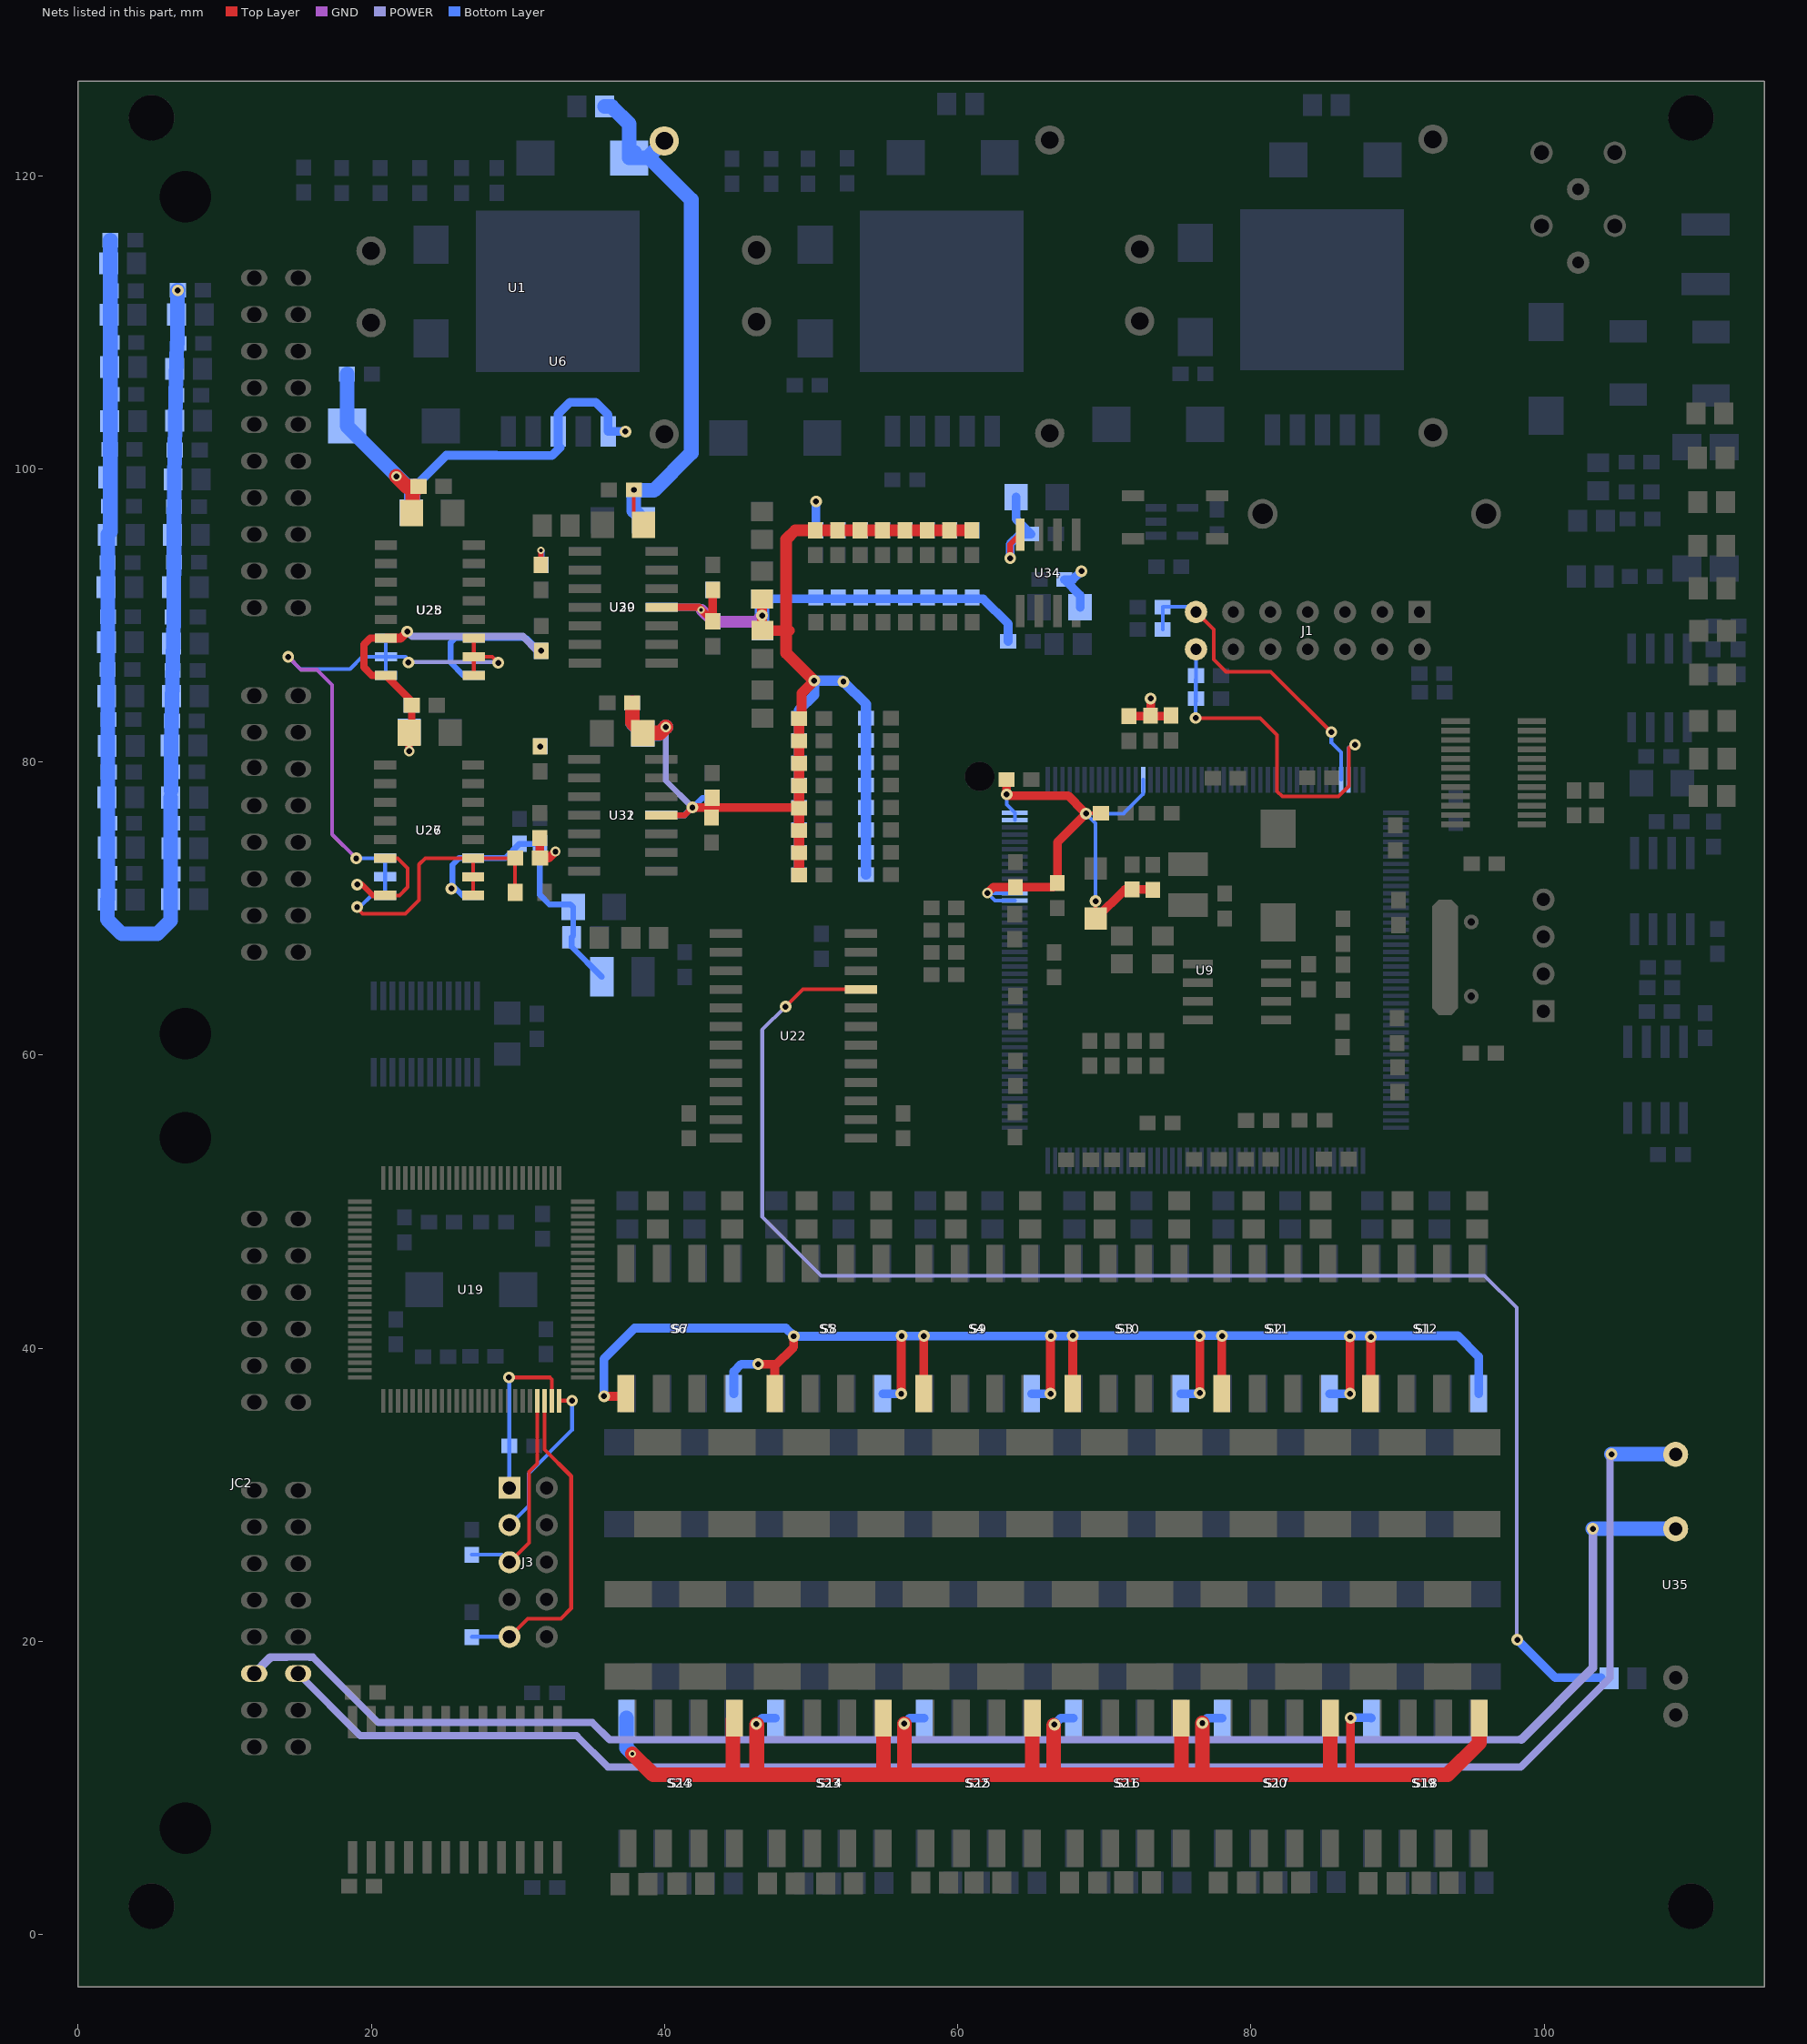
[diagram p0: the nets of this part, all layers, seen from the top]
# Altium PCB MISC86180.PCBDOC (part 6 of 9)
Units mm, origin at the board's own origin, x right, y up, seen from the top; angles counter-clockwise.
Board outline 115 x 130 mm, 4 copper layers (Top Layer, GND, POWER, Bottom Layer); 475 components, 355 nets, 1755 pads, 459 vias.

## Via types
v1: diameter 0.8, hole 0.4, Top Layer to Bottom Layer, 339 vias
v2: diameter 0.7, hole 0.4, Top Layer to Bottom Layer, 83 vias
v3: diameter 0.5, hole 0.254, Top Layer to Bottom Layer, 37 vias

## Nets (pads, with @x,y where several pads share a name; then routed paths per layer and width w, separated by ;. In a path a pad name is that pad's centre, name@x,y a point inside that pad or via, vN(x,y) a via of type N, cw(c..) or ccw(c..) an arc to the next point about the centre after c; other vN are vias at no path point) (continued)
CT26: R104.2 U22.9 | length 104
  Top Layer w0.254: v1(48.25,63.31) 49.429,64.489 U22.9@53.392,64.489
  POWER w0.254: v1(48.25,63.31) 46.66,61.72 46.66,48.99 50.69,44.96 95.92,44.96 98.11,42.77 v1@98.11,20.11
  Bottom Layer w0.6: v1@98.19,20.09 100.74,17.54 R104.2@103.879,17.54
  other v1: 98.16,20.12
CTCK: J3.1 R83.2 U19.24 | length 12
  Top Layer w0.254: v1(29.39,38.01) 32.19,38.01 32.316,37.884 U19.24@32.316,36.414
  Bottom Layer w0.254: v1(29.39,38.01) 29.41,37.99 R83.2@29.41,33.332 J3.1@29.41,30.5
CTDI: J3.9 R85.2 U19.23 | length 22.5
  Top Layer w0.254: J3.9@29.425,20.325 30.659,21.56 32.93,21.56 33.63,22.26 33.63,31.28 31.816,33.094 U19.23@31.816,36.414
  Bottom Layer w0.254: R85.2@26.848,20.3 26.874,20.325 J3.9@29.425,20.325
CTDO: J3.3 U19.25 | length 11.1
  Top Layer w0.254: U19.25@32.816,36.414 32.832,36.43 v1(33.69,36.43)
  Bottom Layer w0.254: J3.3@29.425,27.945 30.719,29.24 30.719,31.46 33.69,34.431 v1(33.69,36.43)
CTMS: J3.5 R84.2 U19.22 | length 14.6
  Top Layer w0.254: J3.5@29.425,25.405 30.76,26.741 30.76,31.58 31.316,32.136 U19.22@31.316,36.414
  Bottom Layer w0.254: R84.2@26.848,25.92 28.91,25.92 J3.5@29.425,25.405
CTOUT25: L1.2 R105.2 U25.9 U25.10 U25.11 U26.9 U26.10 U26.11 U27.9 U27.10 U27.11 U28.9 U28.10 U28.11 | length 64.2
  Top Layer w0.254: v1(19.03,70.1) 19.03,70.03 19.415,69.645 22.325,69.645 23.253,70.573 23.253,73.013 23.677,73.437 U27.11@26.934,73.437 ; U27.9@26.934,70.897 U27.10@26.934,72.167 U27.11@26.934,73.437 ; U25.9@26.991,85.91 U25.10@26.991,87.18 ; U25.11@26.991,88.45 U25.10@26.991,87.18 ; v1(28.66,86.77) 28.25,87.18 U25.10@26.991,87.18 ; L1.2@29.815,71.108 29.81,71.113 R105.2@29.81,73.448 29.799,73.437 U27.11@26.934,73.437
  GND w0.254: v1(14.33,87.17) 15.21,86.29 16.29,86.29 17.33,85.25 17.33,75.06 v1(18.97,73.42)
  POWER w0.254: v1(22.53,86.79) 22.56,86.82 28.61,86.82 v1(28.66,86.77)
  Bottom Layer w0.254: v1(14.33,87.17) 15.15,86.35 18.55,86.35 19.377,87.177 U28.10@20.998,87.177 ; v1(18.97,73.42) 18.99,73.44 U26.11@20.941,73.44 U26.10@20.941,72.17 U26.9@20.941,70.9 20.911,70.93 20.04,70.93 19.21,70.1 v1(19.03,70.1) ; U28.9@20.998,85.907 U28.10@20.998,87.177 ; U28.11@20.998,88.447 U28.10@20.998,87.177 ; v1(22.53,86.79) 22.53,86.98 22.333,87.177 U28.10@20.998,87.177
DOUT+: JC2.24 U35.4 | length 114.3
  POWER w0.254: v1@104.48,32.68 v1(104.58,32.78)
  POWER w0.5: JC2.24@15.01,17.814 19.257,13.567 34.003,13.567 36.14,11.43 98.4,11.43 104.48,17.51 v1@104.48,32.68
  Bottom Layer w0.6: U35.4@108.941,32.78 U35.4@108.956,32.765
  Bottom Layer w1: v1(104.58,32.78) U35.4@108.941,32.78
DOUT-: JC2.32 U35.3 | length 111.3
  POWER w0.254: 35.028,14.465 35.078,14.465
  POWER w0.5: 13.14,18.89 13.18,18.93 14.211,18.93 14.217,18.935 15.803,18.935 15.809,18.93 16.01,18.93 20.475,14.465 35.028,14.465 ; 35.078,14.465 36.253,13.29 98.38,13.29 98.42,13.33
  POWER w0.6: JC2.32@12.01,17.814 13.086,18.89 13.14,18.89 ; 98.42,13.33 98.45,13.33 103.31,18.19 v1(103.31,27.685)
  Bottom Layer w1: v1(103.31,27.685) U35.3@108.956,27.685
EMU0: C53.2 J1.13 R6.2 U9.85 | length 21.3
  Top Layer w0.254: J1.13@76.246,90.233 77.449,89.03 77.449,86.981 78.28,86.15 81.34,86.15 85.48,82.01 v1(85.48,82.04)
  Bottom Layer w0.254: R6.2@73.972,89.032 C53.2@73.972,90.556 73.996,90.58 75.899,90.58 J1.13@76.246,90.233 ; v1(85.48,82.04) 85.48,81.31 86.139,80.651 U9.85@86.139,78.793
EMU1: C54.2 J1.14 R7.2 U9.86 | length 25.7
  Top Layer w0.254: v1(76.22,83) 80.62,83 81.77,81.85 81.77,78 82.13,77.64 85.96,77.64 86.67,78.35 86.67,80.98 86.86,81.17 v1(87.09,81.17)
  Bottom Layer w0.254: v1@76.21,83.01 76.21,84.112 76.23,84.132 C54.2@76.23,85.622 ; C54.2@76.246,85.638 J1.14@76.246,87.693 ; U9.86@86.639,78.793 86.639,80.958 86.852,81.17 v1(87.09,81.17)
GNDA: C3.2 C4.1 C15.2 C16.1 C46.1 C47.1 C48.1 C100.1 C101.1 C102.1 C103.1 C104.1 C105.1 C106.1 C107.1 C108.1 C109.1 C110.1 C111.1 C112.1 C113.1 C114.1 C115.1 C116.1 C117.1 C118.1 C119.1 C120.1 C121.1 C122.1 C123.1 C124.1 C126.1 C128.1 C129.1 C130.1 C131.1 C132.1 C133.1 C134.1 C135.1 C136.1 C137.1 C138.1 C139.1 C140.1 C141.1 C142.1 C143.1 C144.1 C145.1 C146.1 C147.1 C148.1 C149.1 C150.1 C151.1 C152.1 C153.1 C154.1 C155.1 C156.1 C157.1 C158.1 C159.1 C160.1 C161.1 C162.1 C163.1 C164.1 C165.1 C166.1 C167.1 C168.1 C169.1 C170.1 C171.1 C172.1 C173.1 C174.1 C175.1 C176.1 C177.1 C178.1 C179.1 C180.1 C181.1 C182.1 C183.1 C184.1 C185.1 C186.1 C187.1 C188.1 C189.1 C191.1 C192.1 C195.1 C196.1 C197.1 C199.1 C200.1 C201.1 C202.1 C203.1 C204.1 C205.1 C206.1 C208.1 C209.1 L2.2 R105.1 R106.2 R107.2 R108.2 R109.2 R110.2 R111.2 R112.2 R113.2 R114.2 R115.2 R116.2 R117.2 R118.2 R119.2 R120.2 R121.2 R122.2 R123.2 R124.2 R125.2 R126.2 R127.2 R128.2 R129.2 R130.2 R132.2 R134.2 R137.1 R139.1 R141.1 R143.1 R145.1 R147.1 R149.1 R151.1 R153.1 R155.1 R157.1 R159.1 R161.1 R163.1 R165.1 R167.1 R173.2 R181.2 S1.5 S2.5 S3.5 S4.5 S5.5 S6.5 S7.5 S8.5 S9.5 S10.5 S11.5 S12.5 S13.5 S14.5 S15.5 S16.5 S17.5 S18.5 S19.5 S20.5 S21.5 S22.5 S23.5 S24.5 U1.4 U6.1 U6.3 U9.32 U9.33 U9.43 U9.44 U9.58 U25.6 U25.8 U26.6 U26.8 U27.6 U27.8 U28.6 U28.8 U29.11 U30.11 U31.11 U32.11 U34.4 | length 686.3
  Top Layer w0.254: 20.24,85.94 U25.8@20.96,85.94 ; U27.8@20.934,70.897 21.907,70.897 22.47,71.46 22.47,72.75 21.783,73.437 U27.6@20.934,73.437 ; v1@22.34,88.79 v1(22.45,88.9) ; C129.1@22.739,96.992 C129.1@22.809,97.061 ; R105.1@31.488,73.47 R105.1@31.51,73.448 ; S6.5@37.185,36.73 S6.5@37.357,36.902 ; v1(37.904,98.564) 37.904,96.823 C132.1@38.565,96.162 ; 43.218,76.9 43.248,76.87 43.248,76.9 C178.1@43.248,77.552 ; S13.5@44.763,14.681 S13.5@44.763,14.774 ; v1@46.16,14.37 v1(46.26,14.37) v1@46.26,14.34 ; R137.1@50.284,95.804 R139.1@51.808,95.804 R141.1@53.332,95.804 R143.1@54.856,95.804 R145.1@56.38,95.804 R147.1@57.904,95.804 R149.1@59.428,95.804 ; S14.5@54.923,14.637 S14.5@54.923,14.774 ; v1@56.14,40.82 v1@56.14,40.85 ; v1@63.32,77.8 v1(63.33,77.79) ; 66.54,10.91 66.54,11.09 ; v1@68.59,76.63 v1(68.74,76.48) 68.752,76.492 C204.1@69.76,76.492 ; C46.1@69.4,69.307 v1(69.4,70.51) ; C47.1@73.288,71.3 C47.1@73.308,71.28 ; S17.5@85.2,14.571 S17.5@85.403,14.774 S17.5@85.403,14.767 ; 86.79,10.98 86.79,11.24
  Top Layer w0.4: v1(19.04,71.64) 19.35,71.64 20.093,70.897 U27.8@20.934,70.897 ; v2@22.581,80.739 v2(22.59,80.73) ; C148.1@31.568,93.508 C148.1@31.568,93.438 v3@31.568,94.432 ; U31.11@39.764,76.365 41.365,76.365 v1(41.9,76.9) ; v1(63.57,93.9) 63.57,94.849 64.228,95.507 U34.4@64.253,95.507
  Top Layer w0.5: U25.6@20.991,88.45 19.93,88.45 19.49,88.01 19.49,86.46 20.04,85.91 U25.8@20.991,85.91 C141.1@22.76,84.14 ; v2@22.581,80.739 C130.1@22.581,82.006 22.76,82.185 C141.1@22.76,83.872 ; U29.11@39.804,90.551 42.326,90.551 C151.1@43.282,89.596 C151.1@43.282,89.562
  Top Layer w0.6: U25.6@20.991,88.45 22,88.45 v1@22.34,88.79 ; R105.1@31.488,73.47 C169.1@31.488,74.81 ; R105.1@31.51,73.448 32.118,73.448 v2(32.56,73.89) ; v1(35.87,36.73) S6.5@37.185,36.73 ; v1(41.9,76.9) 43.218,76.9 ; C175.1@43.212,76.21 43.218,76.216 43.218,76.9 ; C151.1@43.288,89.602 C154.1@43.288,91.738 ; v1(46.38,38.92) 47.517,38.92 ; S5.5@47.517,36.902 47.517,38.797 48.81,40.09 v1(48.81,40.82) ; R161.1@49.168,76.856 49.124,76.9 43.248,76.9 43.218,76.9 ; v1(56.14,36.9) v1@56.14,40.82 ; S4.5@57.677,36.902 v1@57.677,40.847 ; v2(62.02,71.06) 62.428,71.468 C201.1@63.918,71.468 66.52,71.468 C202.1@66.792,71.74 66.792,74.532 v1(68.74,76.48) ; v1@63.32,77.8 C203.1@63.32,78.802 ; v1(63.33,77.79) 63.418,77.702 67.518,77.702 v1@68.59,76.63 ; v1(66.322,36.902) v1@66.322,40.822 ; S3.5@67.837,36.902 v1@67.837,40.857 ; C46.1@69.4,69.307 71.393,71.3 C48.1@71.888,71.3 C47.1@73.288,71.3 ; C200.1@71.672,83.13 R181.2@74.508,83.13 ; v1(73.15,84.33) 73.152,84.328 C199.1@73.152,83.15 ; v1(76.5,36.954) v1@76.5,40.83 ; S2.5@77.997,36.902 v1@77.997,40.817 ; v1(86.75,36.9) v1@86.75,40.81 ; 86.79,11.24 v1(86.79,14.8) ; S1.5@88.157,36.902 v1@88.157,40.767
  Top Layer w0.7: R134.2@46.65,91.111 v1(46.65,89.99) 46.65,89.002 R132.2@46.686,88.965 48.525,88.965 ; R167.1@49.168,72.284 R165.1@49.168,73.808 R163.1@49.168,75.332 R161.1@49.168,76.856 R159.1@49.168,78.38 R157.1@49.168,79.904 R155.1@49.168,81.428 R153.1@49.168,82.952 49.34,83.124 49.34,84.68 v1(50.21,85.55)
  Top Layer w0.8: v1(50.21,85.55) 50.18,85.55 48.3,87.43 48.3,95.2 48.904,95.804 R137.1@50.284,95.804 R139.1@51.808,95.804 R141.1@53.332,95.804 R143.1@54.856,95.804 R145.1@56.38,95.804 R147.1@57.904,95.804 R149.1@59.428,95.804 R151.1@60.952,95.804
  Top Layer w1: v2(21.71,99.49) 22.402,98.798 C140.1@23.22,98.798 22.809,98.386 C129.1@22.809,97.061 ; C138.1@37.794,84.048 37.794,82.707 C134.1@38.525,81.976 39.676,81.976 v2(40.08,82.38) ; v3(37.81,12.33) 39.23,10.91 44.67,10.91 ; S13.5@44.67,14.681 44.67,10.91 ; v1@46.29,14.34 46.29,10.91 ; 54.923,11.047 S14.5@54.923,14.774 ; 55.06,11.047 55.06,10.91 ; v1@56.35,14.38 56.35,10.91 ; 65.083,10.933 S15.5@65.083,14.774 ; 66.54,11.09 v1@66.54,14.28 ; 75.243,10.917 S16.5@75.243,14.774 ; 76.68,10.95 v1(76.68,14.43) ; S17.5@85.41,14.767 85.41,10.91 ; S18.5@95.563,14.774 95.563,13.073 93.4,10.91 85.41,10.91 ; 44.67,10.91 46.29,10.91 ; 46.29,10.91 55.06,10.91 ; 55.06,10.91 56.35,10.91 ; 56.35,10.91 66.54,10.91 85.41,10.91
  GND w0.8: v3@42.51,90.39 43.338,89.562 46.222,89.562 v1(46.65,89.99)
  POWER w0.4: v2(40.08,82.38) 40.08,78.72 v1(41.9,76.9)
  POWER w0.5: v1(22.45,88.9) 22.79,88.56 30.342,88.56 31.312,87.59 v1(31.582,87.59)
  Bottom Layer w0.254: C131.1@23.22,97.499 C142.1@23.22,98.834 ; R173.2@33.661,68.052 R173.2@33.769,68.16 ; C166.1@43.252,89.662 C163.1@43.252,91.738 ; C126.1@46.65,88.983 C126.1@46.686,88.947 ; C149.1@51.844,95.804 C152.1@53.368,95.804 C155.1@54.892,95.804 C158.1@56.416,95.804 C161.1@57.94,95.804 C164.1@59.464,95.804 ; v2(62.02,71.06) v2@62.037,71.043 ; v1(63.33,77.79) 63.33,77.103 U9.44@63.889,76.543 U9.43@63.889,76.043 ; U9.32@63.889,70.543 63.883,70.55 62.53,70.55 v2@62.037,71.043 ; U9.33@63.889,71.043 v2@62.037,71.043 ; v1(69.4,70.51) 69.4,75.82 v1(68.74,76.48) 71.296,76.48 72.639,77.823 U9.58@72.639,78.793
  Bottom Layer w0.4: v2(22.59,80.73) 22.581,80.739 C143.1@22.581,82.042 22.74,82.201 C144.1@22.74,83.868 ; v1(25.46,71.36) 25.53,71.43 25.53,71.91 ; U26.8@26.941,70.9 26.21,70.9 25.53,71.58 25.53,71.91 ; U28.8@26.998,85.907 26.283,85.907 25.41,86.78 25.41,88.14 25.717,88.447 U28.6@26.998,88.447 30.593,88.447 31.464,87.576 C160.1@31.568,87.576 v1(31.582,87.59) ; C184.1@31.502,74.47 C184.1@31.502,74.37 ; v1(31.524,81.056) C181.1@31.524,81.072 ; v3(31.56,94.44) 31.604,94.396 C157.1@31.604,93.438 ; L2.2@35.725,65.335 33.661,67.399 R173.2@33.661,68.052 33.769,68.16 C208.1@33.769,70.098 33.577,70.29 32.14,70.29 31.502,70.928 C184.1@31.502,74.37 ; U32.11@39.764,76.375 41.375,76.375 v1(41.9,76.9) 41.94,76.9 42.592,77.552 C187.1@43.212,77.552 ; 25.53,71.91 25.53,72.99 25.98,73.44 U26.6@26.941,73.44 29.121,73.44 C209.1@30.102,74.42 31.452,74.42 C184.1@31.502,74.37
  Bottom Layer w0.5: U30.11@39.804,90.561 42.354,90.561 43.252,89.662 C166.1@43.318,89.596
  Bottom Layer w0.6: C142.1@23.22,98.834 23.22,99.033 25.107,100.92 28.544,100.92 28.558,100.905 32.325,100.905 32.87,101.45 32.747,101.573 U6.3@32.747,102.555 32.747,103.737 33.55,104.54 35.29,104.54 36.147,103.683 U6.1@36.147,102.555 37.315,102.555 v1(37.33,102.54) ; v1(35.87,36.73) 35.87,39.29 37.96,41.38 48.27,41.38 v1@48.81,40.84 ; S7.5@44.723,36.902 44.723,38.413 45.23,38.92 v1(46.38,38.92) ; v1(46.26,14.37) 46.664,14.774 S23.5@47.557,14.774 ; C128.1@46.65,91.129 53.368,91.129 61.731,91.129 63.43,89.43 C197.1@63.43,88.228 ; v1(48.81,40.82) v1@56.17,40.82 ; v1(50.33,97.77) 50.32,97.76 C146.1@50.32,95.804 C149.1@51.844,95.804 C152.1@53.368,95.804 C155.1@54.892,95.804 C158.1@56.416,95.804 C161.1@57.94,95.804 C164.1@59.464,95.804 C167.1@60.988,95.804 ; S8.5@54.883,36.902 v1@56.138,36.902 ; v1@56.21,40.84 v1@67.84,40.84 ; v1(56.34,14.39) 56.724,14.774 S22.5@57.717,14.774 ; v1(63.57,93.9) 63.57,94.86 64.258,95.548 C206.1@64.99,95.548 63.979,96.559 C205.1@63.979,98.068 ; S9.5@65.043,36.902 v1(66.322,36.902) ; v1(66.59,14.33) 67.034,14.774 S21.5@67.877,14.774 ; v1(67.84,40.86) v1@86.82,40.86 ; C195.1@68.341,90.552 68.341,91.371 C196.1@67.27,92.442 67.852,92.442 v1(68.43,93.02) ; S10.5@75.203,36.902 v1@76.448,36.902 ; v1(76.68,14.43) 77.024,14.774 S20.5@78.037,14.774 ; S11.5@85.363,36.902 v1@86.748,36.902 ; v1(86.79,14.8) 88.171,14.8 S19.5@88.197,14.774 ; v1@86.83,40.85 94.11,40.85 95.523,39.437 S12.5@95.523,36.902
  Bottom Layer w0.7: C191.1@49.168,72.32 C188.1@49.168,73.844 C185.1@49.168,75.368 C182.1@49.168,76.892 C179.1@49.168,78.416 C176.1@49.168,79.94 C173.1@49.168,81.464 C170.1@49.168,82.988 49.168,83.538 50.21,84.58 v1(50.21,85.55) v1@52.13,85.55 ; v1(52.2,85.48) 53.74,83.94 C171.1@53.74,82.988 C174.1@53.74,81.464 C177.1@53.74,79.94 C180.1@53.74,78.416 C183.1@53.74,76.892 C186.1@53.74,75.368 C189.1@53.74,73.844 C192.1@53.74,72.32
  Bottom Layer w1: C100.1@2.2,115.598 2.2,110.51 2.2,101.318 2.2,95.701 2.02,95.521 C112.1@2.02,93.608 2.02,84.492 2.02,79.31 2.02,74.162 2.02,70.653 R130.2@1.985,70.618 1.985,69.265 2.98,68.27 5.4,68.27 6.321,69.191 R129.2@6.321,70.642 R125.2@6.321,77.572 ; R125.2@6.34,78.061 6.34,81.122 6.52,89.88 6.54,95.502 6.55,99.282 6.64,105.048 C103.1@6.74,108.596 ; C103.1@6.77,108.558 C101.1@6.77,112.18 ; v1(6.8,112.17) 6.81,112.18 C101.1@6.81,112.188 ; C16.1@18.34,106.458 18.34,102.926 C15.2@18.344,102.922 22.432,98.834 C142.1@22.729,98.834 ; C131.1@22.729,97.008 C142.1@22.729,98.343 ; C4.1@35.921,124.712 36.398,124.712 37.586,123.524 C3.2@37.586,121.208 ; S24.5@37.397,14.774 37.397,12.743 v3(37.81,12.33) ; C139.1@37.794,84.012 37.794,82.671 C135.1@38.525,81.94 39.64,81.94 v2(40.08,82.38) ; C3.2@37.968,121.59 C3.2@37.586,121.208 ; C133.1@38.561,96.482 37.904,97.139 C137.1@37.904,98.528 39.268,98.528 41.82,101.08 41.82,118.35 38.962,121.208 C3.2@37.586,121.208 ; U1.4@39.981,122.368 38.821,121.208 C3.2@37.586,121.208 ; C126.1@46.65,88.983 v1(46.65,89.99) C128.1@46.65,91.129
  other v1: 88.17,40.78 86.74,40.82 56.17,40.85 57.68,40.85 66.35,40.85 76.49,40.84 78.02,40.84
  other v3: 42.5,90.37